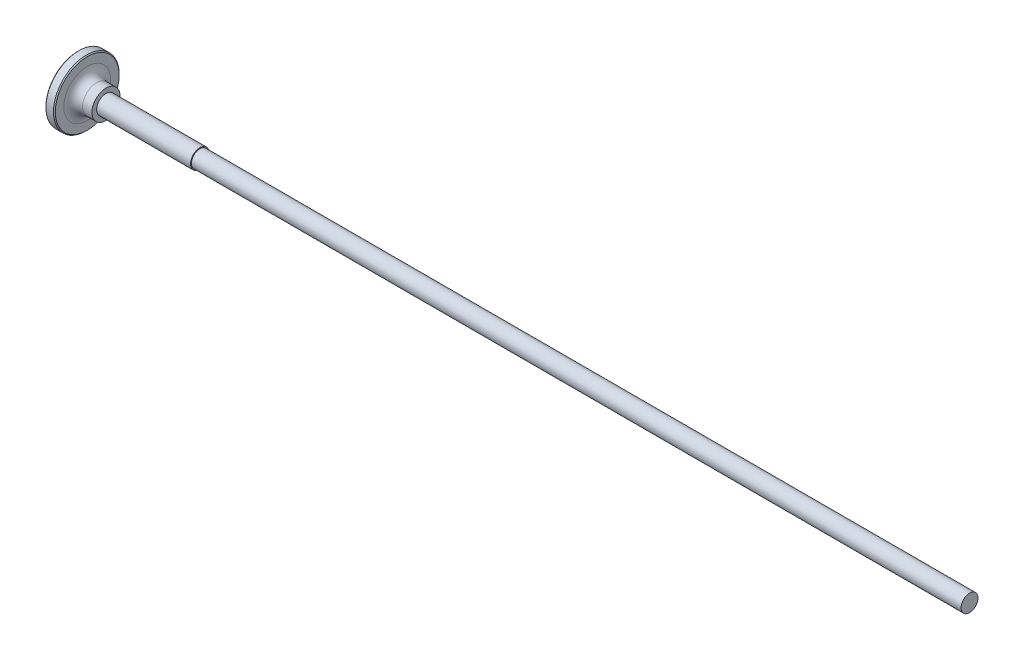
from build123d import *

# Parameters (mm, degrees)
SKETCH_1_R      = 35
EXTRUDE_1_DEPTH = 10
SKETCH_2_R      = 15
EXTRUDE_2_DEPTH = 20
SKETCH_3_R      = 10
EXTRUDE_3_DEPTH = 100
SKETCH_4_R      = 9
EXTRUDE_4_DEPTH = 820
CHAMFER_1_SIZE  = 1
FILLET_1_R      = 10


with BuildPart() as part:
    # 草图1 → 凸台-拉伸1 (new body)
    with BuildSketch(Plane(origin=(0, 0, 0), x_dir=(0, 0, -1), z_dir=(1, 0, 0))):
        Circle(SKETCH_1_R)
    extrude(amount=EXTRUDE_1_DEPTH)

    # 草图2 → 凸台-拉伸2 (add)
    with BuildSketch(Plane(origin=(10, 0, 0), x_dir=(0, 0, -1), z_dir=(1, 0, 0))):
        Circle(SKETCH_2_R)
    extrude(amount=EXTRUDE_2_DEPTH)

    # 草图3 → 凸台-拉伸3 (add)
    with BuildSketch(Plane(origin=(30, 0, 0), x_dir=(0, 0, -1), z_dir=(1, 0, 0))):
        Circle(SKETCH_3_R)
    extrude(amount=EXTRUDE_3_DEPTH)

    # 草图4 → 凸台-拉伸4 (add)
    with BuildSketch(Plane(origin=(130, 0, 0), x_dir=(0, 0, -1), z_dir=(1, 0, 0))):
        with Locations(Location((0, 0, 0), (0, 0, 180))):
            Circle(SKETCH_4_R)
    extrude(amount=EXTRUDE_4_DEPTH)

    # 倒角1
    chamfer_1_edges = [part.edges().sort_by_distance(p)[0] for p in [
        (0, 0, 35),
        (10, 0, 35),
    ]]
    chamfer(chamfer_1_edges, length=CHAMFER_1_SIZE)

    # 圆角1
    fillet_1_edges = [part.edges().sort_by_distance(p)[0] for p in [
        (10, 0, 15),
    ]]
    fillet(fillet_1_edges, radius=FILLET_1_R)


solid = part.part
